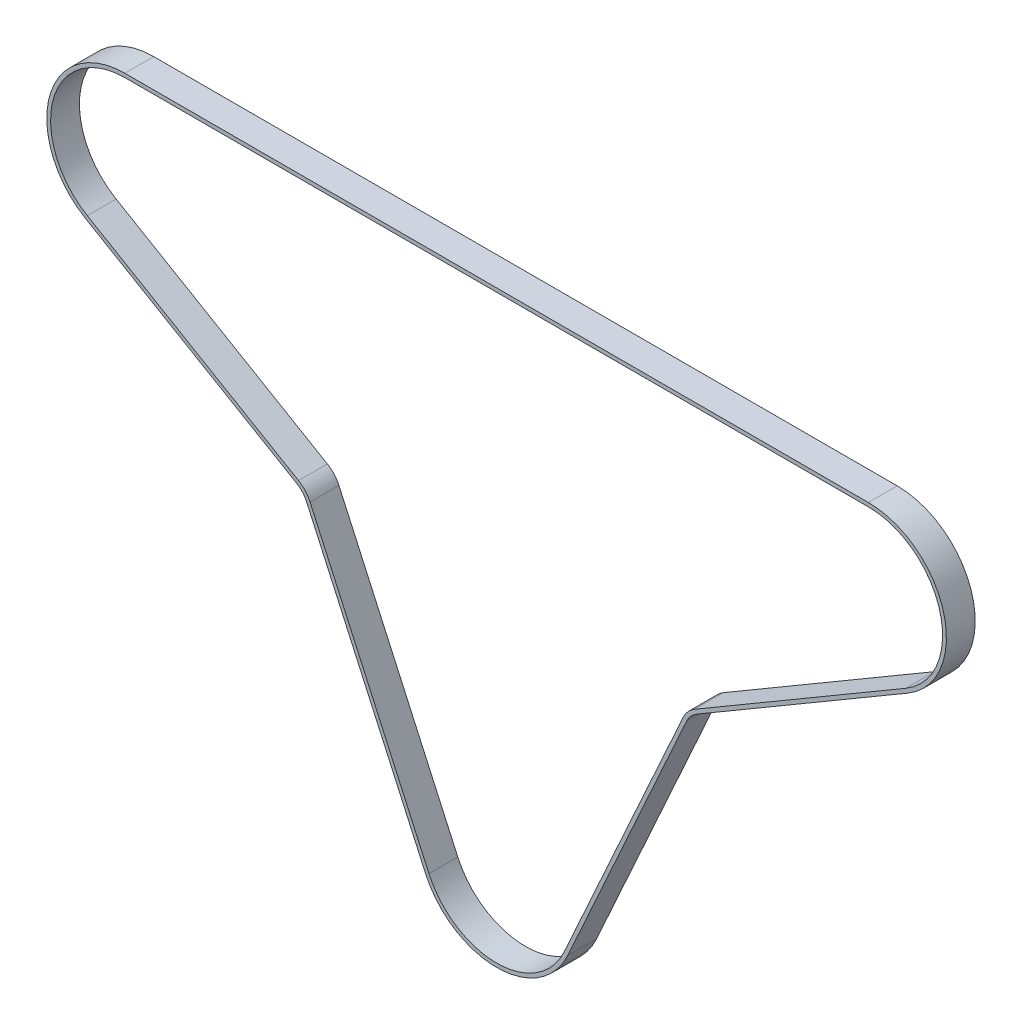
SolidWorks part; units mm, degrees
ref_plane "前视基准面" through (0, 0, 0) normal (0, 0, 1) x (1, 0, 0)
ref_plane "上视基准面" through (0, 0, 0) normal (0, 1, 0) x (1, 0, 0)
ref_plane "右视基准面" through (0, 0, 0) normal (1, 0, 0) x (0, 0, -1)
sketch "草图2" plane through (0, 0, 0) normal (0, 0, 1) x (1, 0, 0)
  line L0 (0, 0) -> (1, 0) construction
  line L1 (0, 0) -> (0, 1) construction
  line L2 (-91.435, -41.422) -> (-248.1189, 304.4428)
  line L3 (-262.3022, 320.1958) -> (-540.7572, 483.3981)
  line L4 (-490, 670.3798) -> (490, 670.3798)
  line L5 (540.7572, 483.3981) -> (262.3022, 320.1958)
  line L6 (248.1189, 304.4428) -> (91.435, -41.422)
  arc A0 (91.435, -41.422) -> (-91.435, -41.422) centre (0, 0) cw
  arc A1 (-248.1189, 304.4428) -> (-262.3022, 320.1958) centre (-280, 290) ccw
  arc A2 (-540.7572, 483.3981) -> (-490, 670.3798) centre (-490, 569.9998) cw
  arc A3 (490, 670.3798) -> (540.7572, 483.3981) centre (490, 569.9998) cw
  arc A4 (262.3022, 320.1958) -> (248.1189, 304.4428) centre (280, 290) ccw
extrude "拉伸-薄壁1" add sketch "草图2" along normal mid plane 38 thin thin type mid plane wall 5
